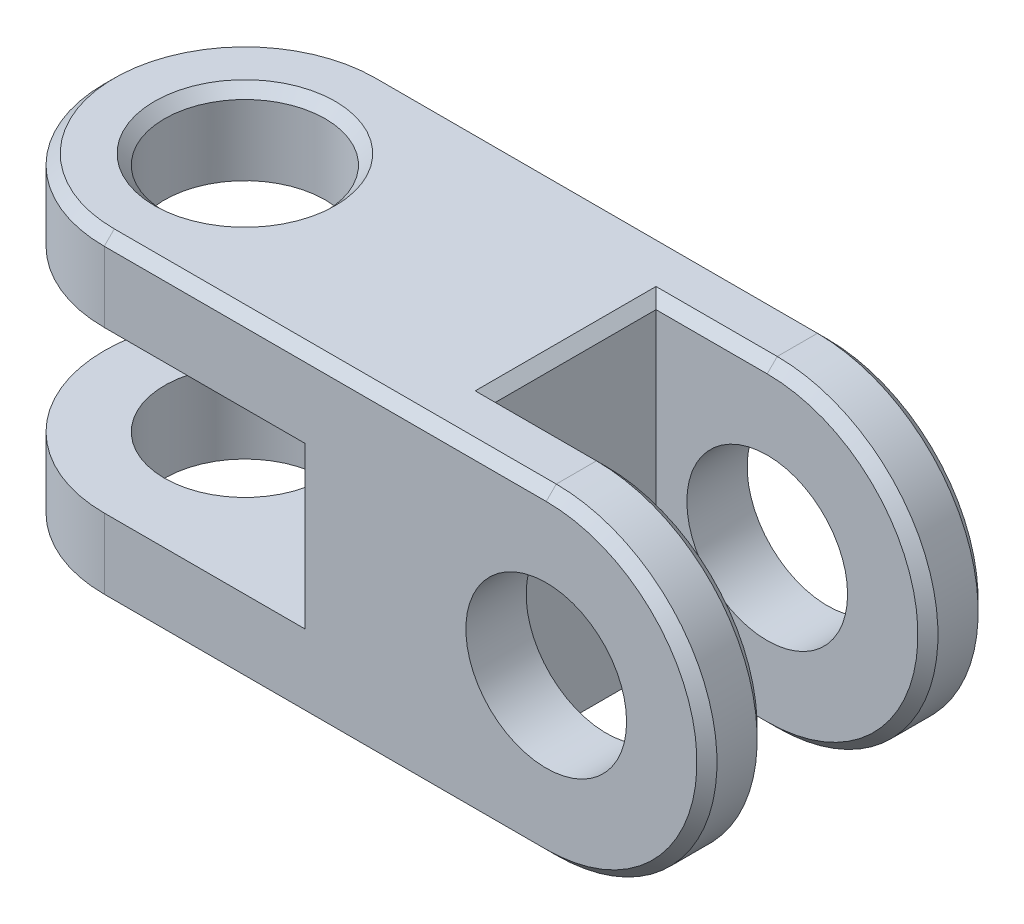
from build123d import *

# Parameters (mm, degrees)
SKETCH1_R               = 4
BOSS_EXTRUDE1_DEPTH     = 16
SKETCH2_W               = 13.535239133
SKETCH2_H               = 8
CUT_EXTRUDE1_DEPTH      = 16
SKETCH3_R               = 4
CUT_EXTRUDE2_DEPTH      = 16
CUT_EXTRUDE3_DEPTH      = 10
CUT_EXTRUDE3_DEPTH_BACK = 16
SKETCH4_W               = 14
SKETCH4_H               = 8
CHAMFER1_SIZE           = 0.5
SCALE1_SCALE            = 0.5


with BuildPart() as part:
    # Sketch1 → Boss-Extrude1 (new body)
    with BuildSketch(Plane(origin=(0, 0, 0), x_dir=(1, 0, 0), z_dir=(0, 1, 0))):
        with BuildLine():
            Line((0, 7), (30, 7))
            Line((30, 7), (30, -7))
            Line((30, -7), (0, -7))
            ThreePointArc((0, -7), (-7, 0), (0, 7))
        make_face()
        with Locations(Location((0, 0, 0), (0, 0, 270))):
            Circle(SKETCH1_R, mode=Mode.SUBTRACT)
    extrude(amount=BOSS_EXTRUDE1_DEPTH)

    # Sketch2 → Cut-Extrude1 (cut)
    with BuildSketch(Plane(origin=(0, 16, 0), x_dir=(1, 0, 0), z_dir=(0, 1, 0))):
        with Locations((23.232380434, 0)):
            Rectangle(SKETCH2_W, SKETCH2_H)
    extrude(amount=-CUT_EXTRUDE1_DEPTH, mode=Mode.SUBTRACT)

    # Sketch3 → Cut-Extrude2 (cut)
    with BuildSketch(Plane.XY.offset(7)):
        with BuildLine():
            Line((30, 16), (22, 16))
            ThreePointArc((22, 16), (27.656854238, 13.656854261), (30, 8.000000031))
            Line((30, 8.000000031), (30, 16))
        make_face()
        with BuildLine():
            Line((30, 0), (30, 8.000000031))
            ThreePointArc((30, 8.000000031), (27.656854261, 2.343145762), (22, 0))
            Line((22, 0), (30, 0))
        make_face()
        with Locations((22, 8)):
            Circle(SKETCH3_R)
    extrude(amount=-CUT_EXTRUDE2_DEPTH, mode=Mode.SUBTRACT)

    # Sketch4 → Cut-Extrude3 (cut, two sides: drawn at the far end of the back side and taken through both)
    with BuildSketch(Plane(origin=(0, 0, 0), x_dir=(0, 0, -1), z_dir=(1, 0, 0)).offset(-CUT_EXTRUDE3_DEPTH_BACK)):
        with Locations((0, 8)):
            Rectangle(SKETCH4_W, SKETCH4_H)
    extrude(amount=CUT_EXTRUDE3_DEPTH + CUT_EXTRUDE3_DEPTH_BACK, mode=Mode.SUBTRACT)

    # Chamfer1
    chamfer1_edges = [part.edges().sort_by_distance(p)[0] for p in [
        (0, 16, -4),
        (19.232380434, 0, 4),
        (16.464760867, 16, 0),
        (19.232380434, 16, 4),
        (19.232380434, 16, -4),
        (30, 8, -4),
        (11, 16, -7),
        (30, 8, 7),
        (-7, 16, 0),
        (30, 8, -7),
        (30, 8, 4),
        (11, 0, 7),
        (-7, 0, 0),
        (11, 0, -7),
        (19.232380434, 0, -4),
        (11, 16, 7),
    ]]
    chamfer(chamfer1_edges, length=CHAMFER1_SIZE)


with BuildPart() as part_1:
    # Scale1: scaled about (0, 0, 0)
    add(part.part.scale(SCALE1_SCALE))


solid = part_1.part
